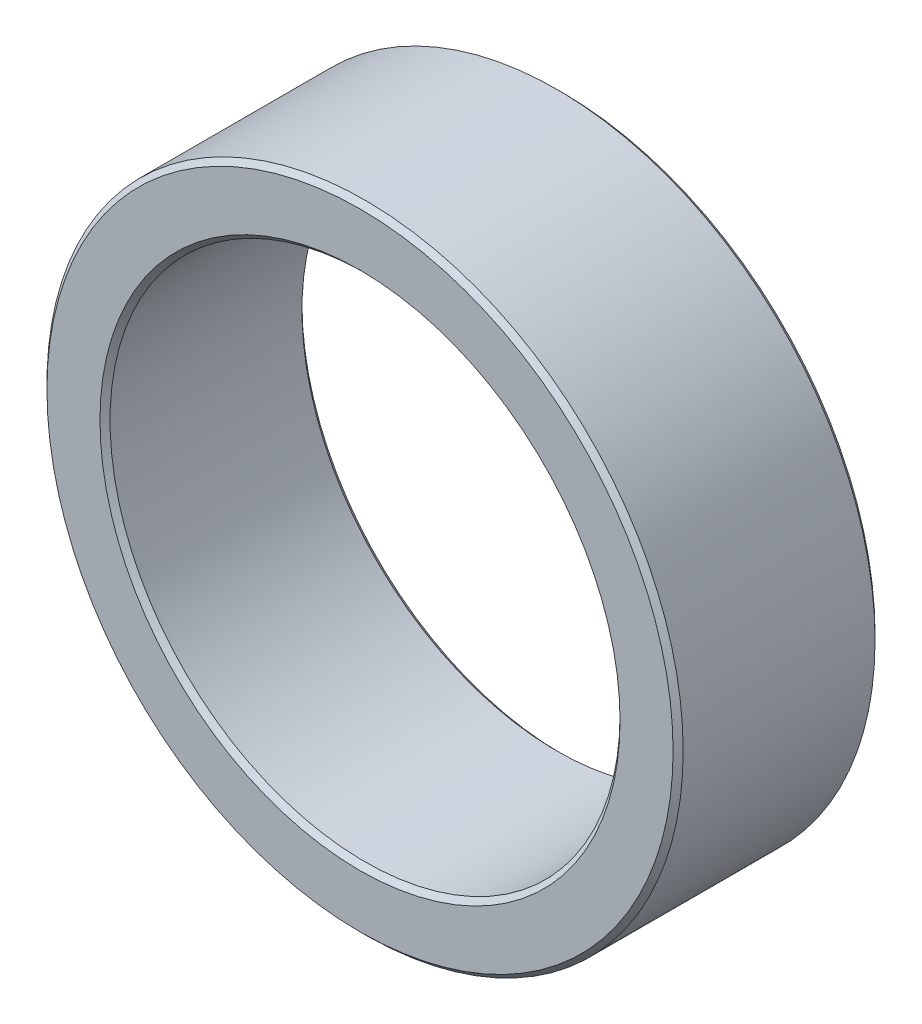
SolidWorks part; units mm, degrees
material "普通碳钢"
ref_plane "前视基准面" through (0, 0, 0) normal (0, 0, 1) x (1, 0, 0)
ref_plane "上视基准面" through (0, 0, 0) normal (0, 1, 0) x (1, 0, 0)
ref_plane "右视基准面" through (0, 0, 0) normal (1, 0, 0) x (0, 0, -1)
sketch "草图1" plane through (0, 0, 0) normal (0, 0, 1) x (1, 0, 0)
  circle A0 centre (0, 0) radius 25.25
  circle A1 centre (0, 0) radius 31.5
  dimension "D1" = 50.5
  dimension "D2" = 63
extrude "凸台-拉伸1" add sketch "草图1" along normal blind 20
chamfer "倒角1" distance 0.5 angle 45 4 edges at (25.25, 0, 0) (31.5, 0, 0) (25.25, 0, 20) (31.5, 0, 20)
